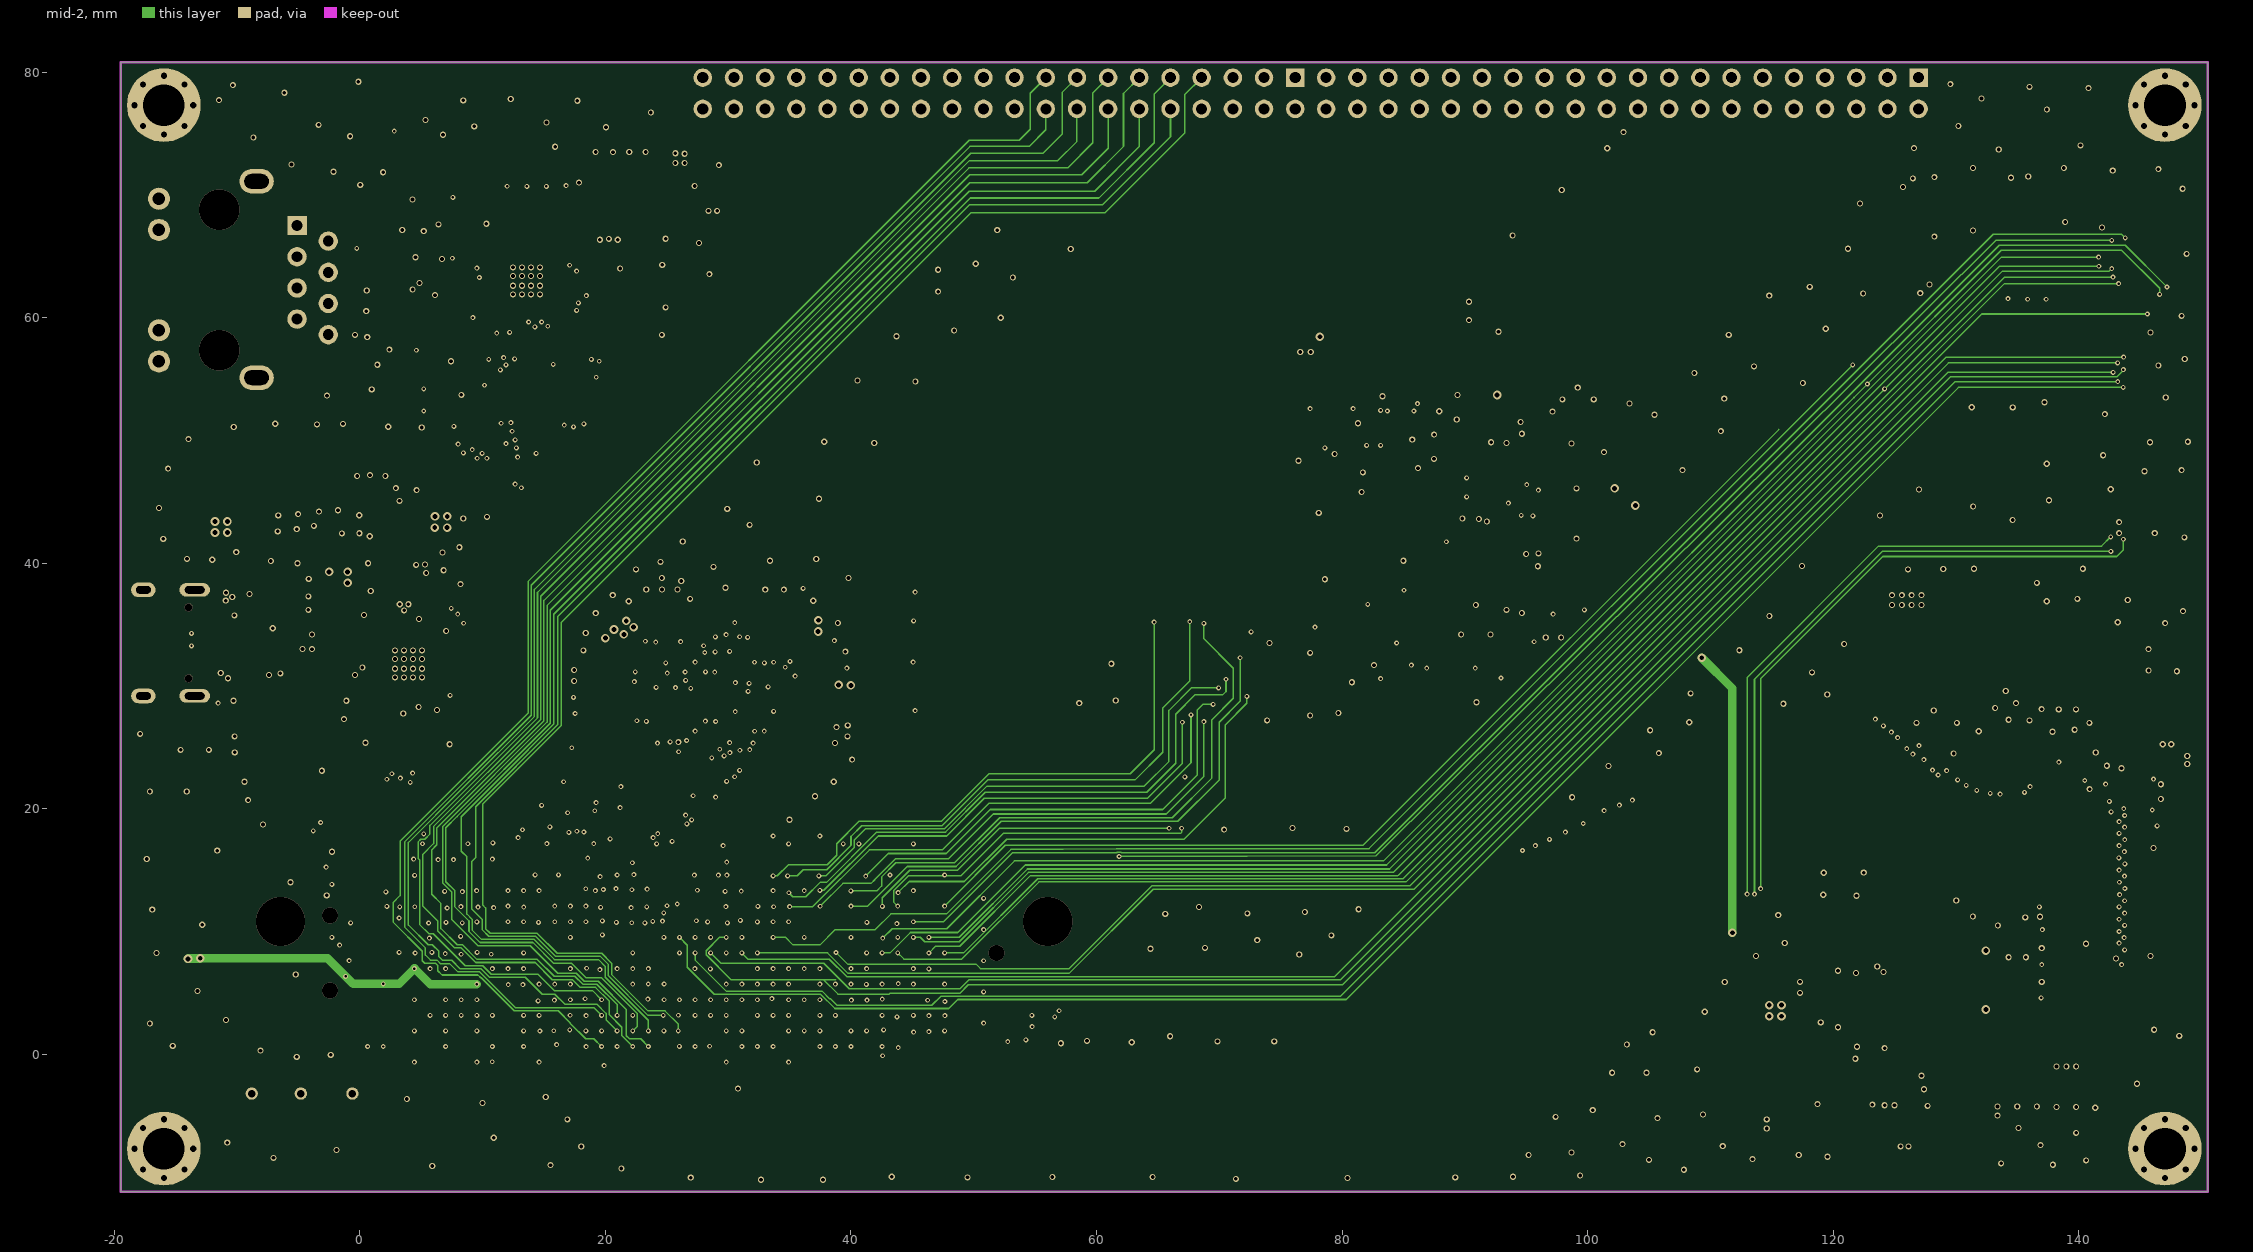
[diagram p0: mid-2]
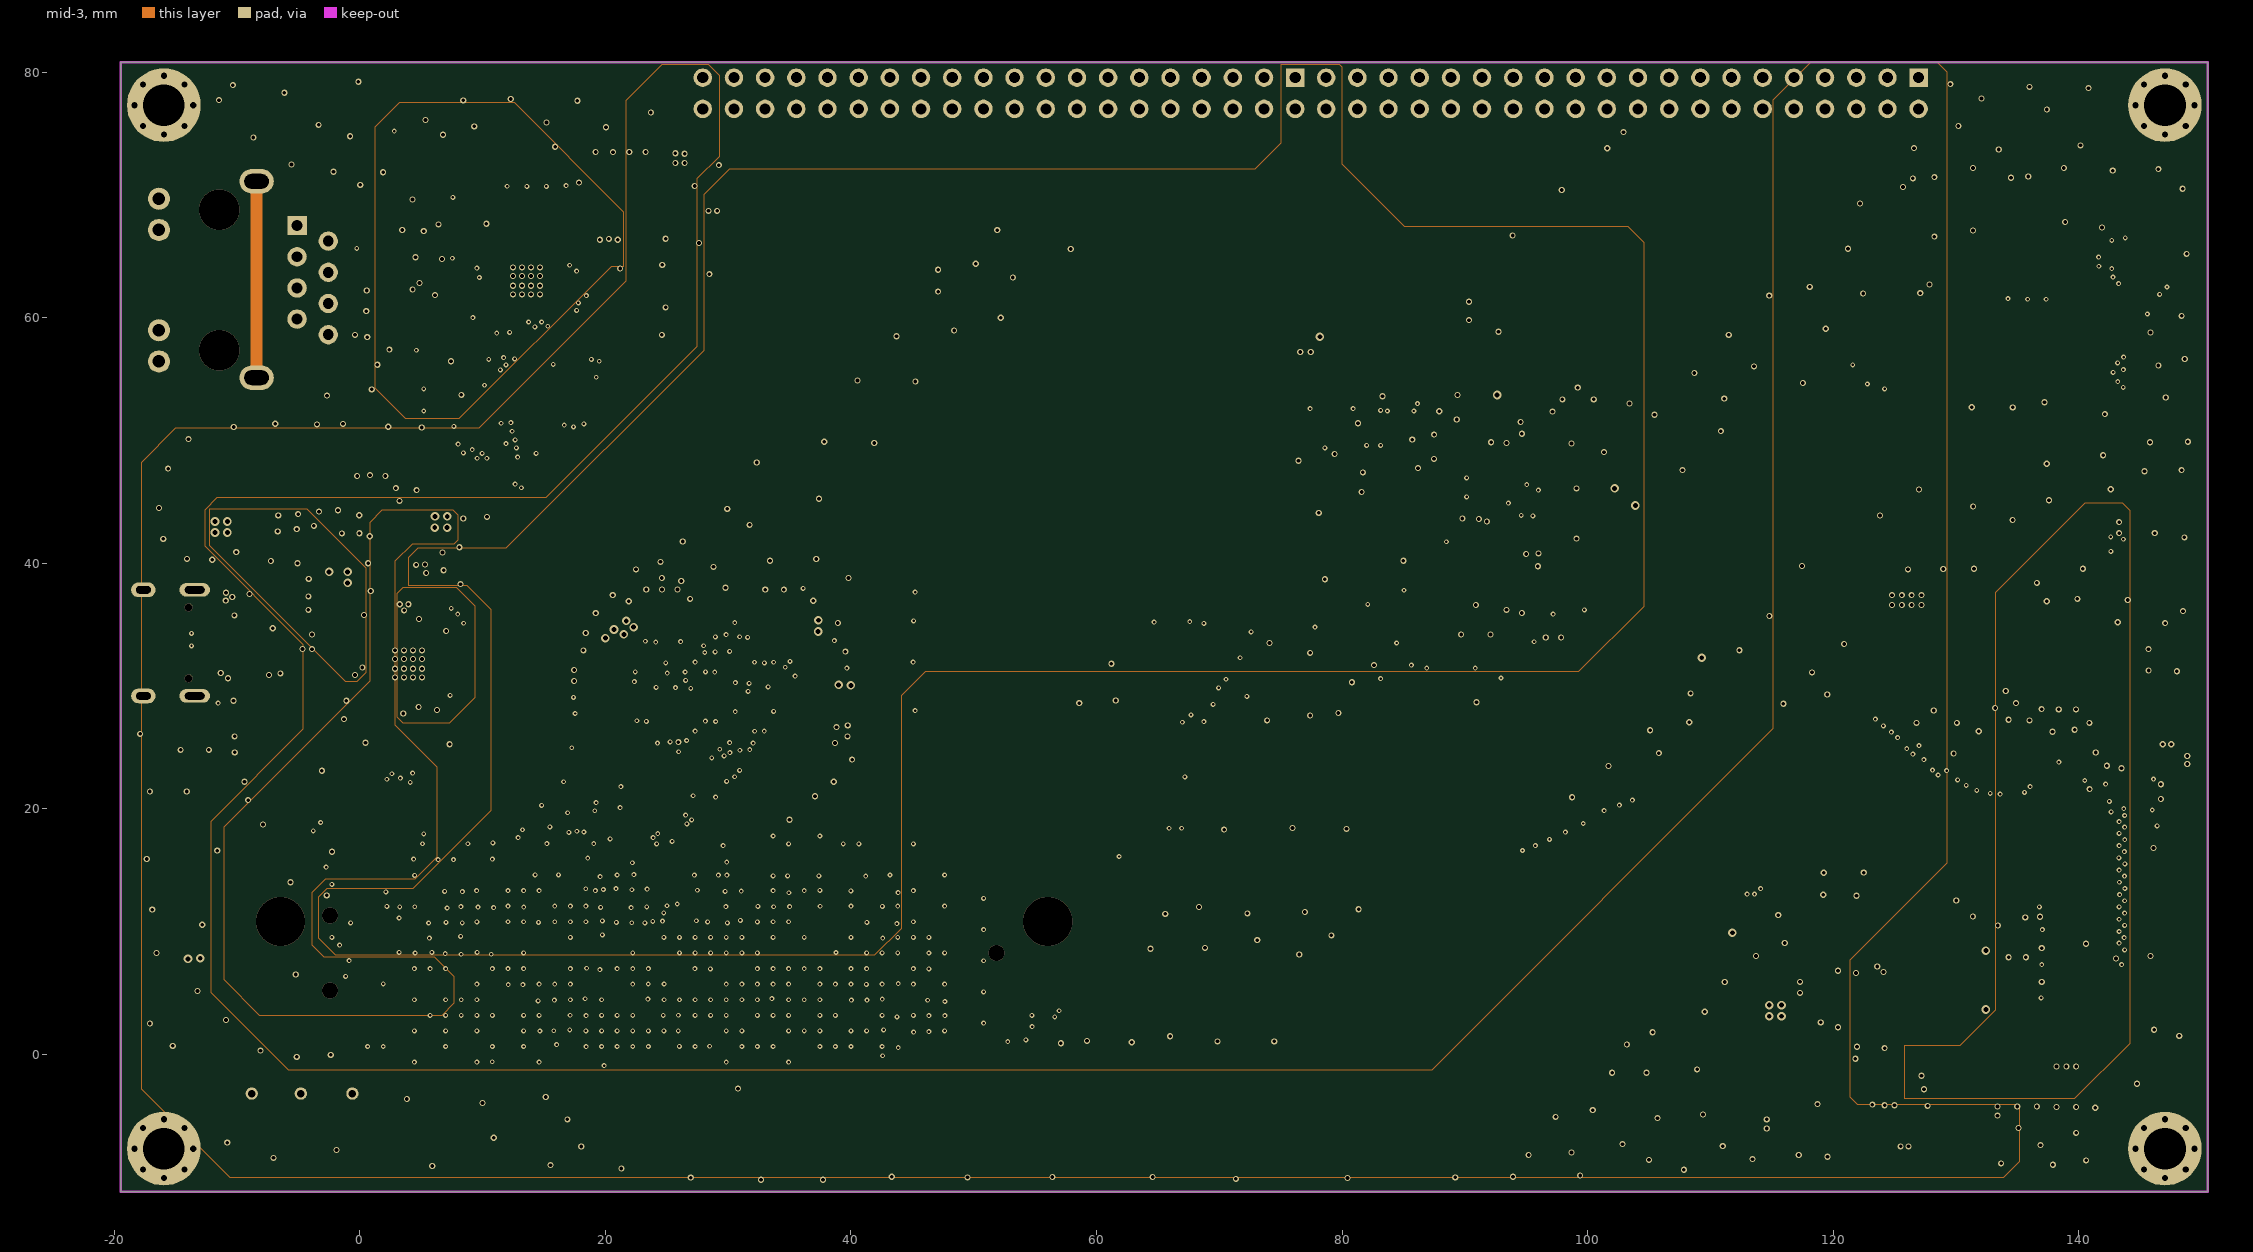
[diagram p1: mid-3]
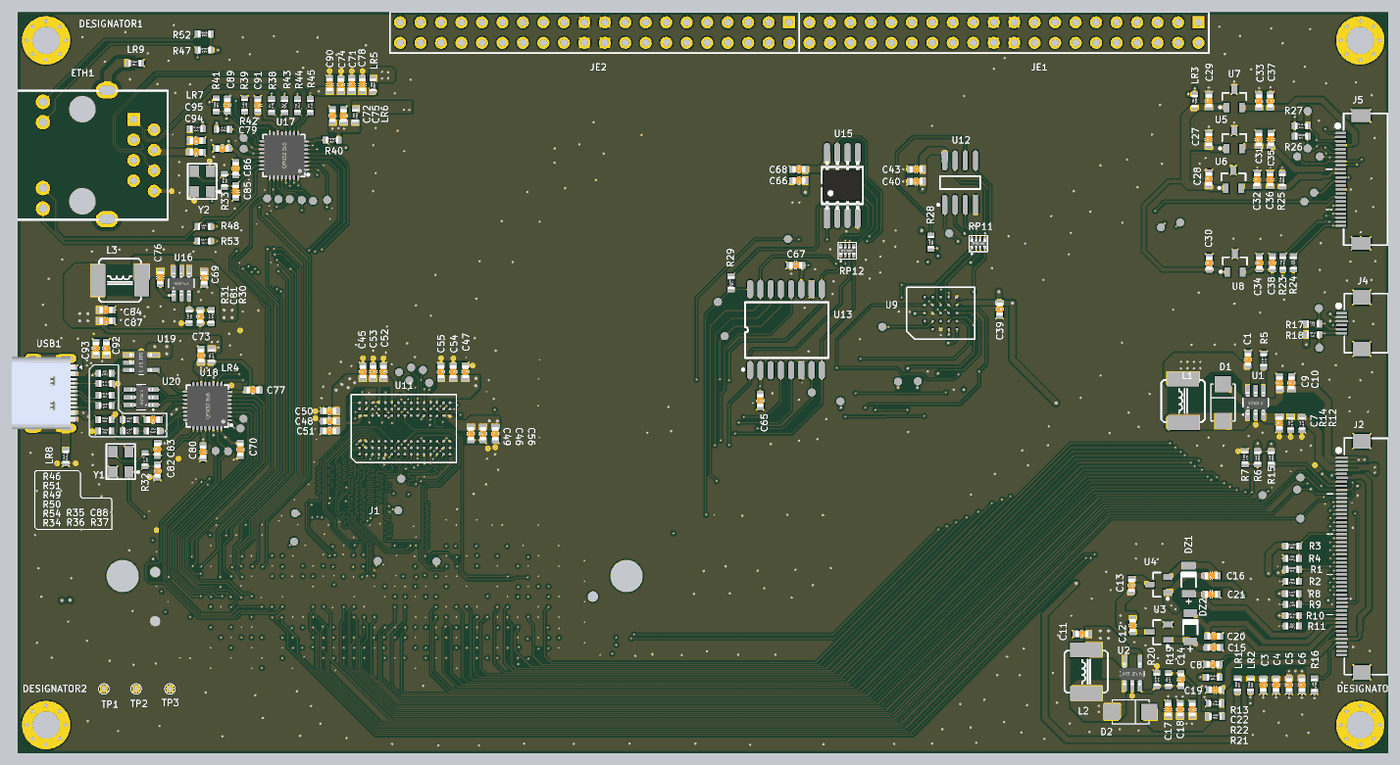
[diagram p2: 3D render of the assembled board from above, using the file's embedded part models]
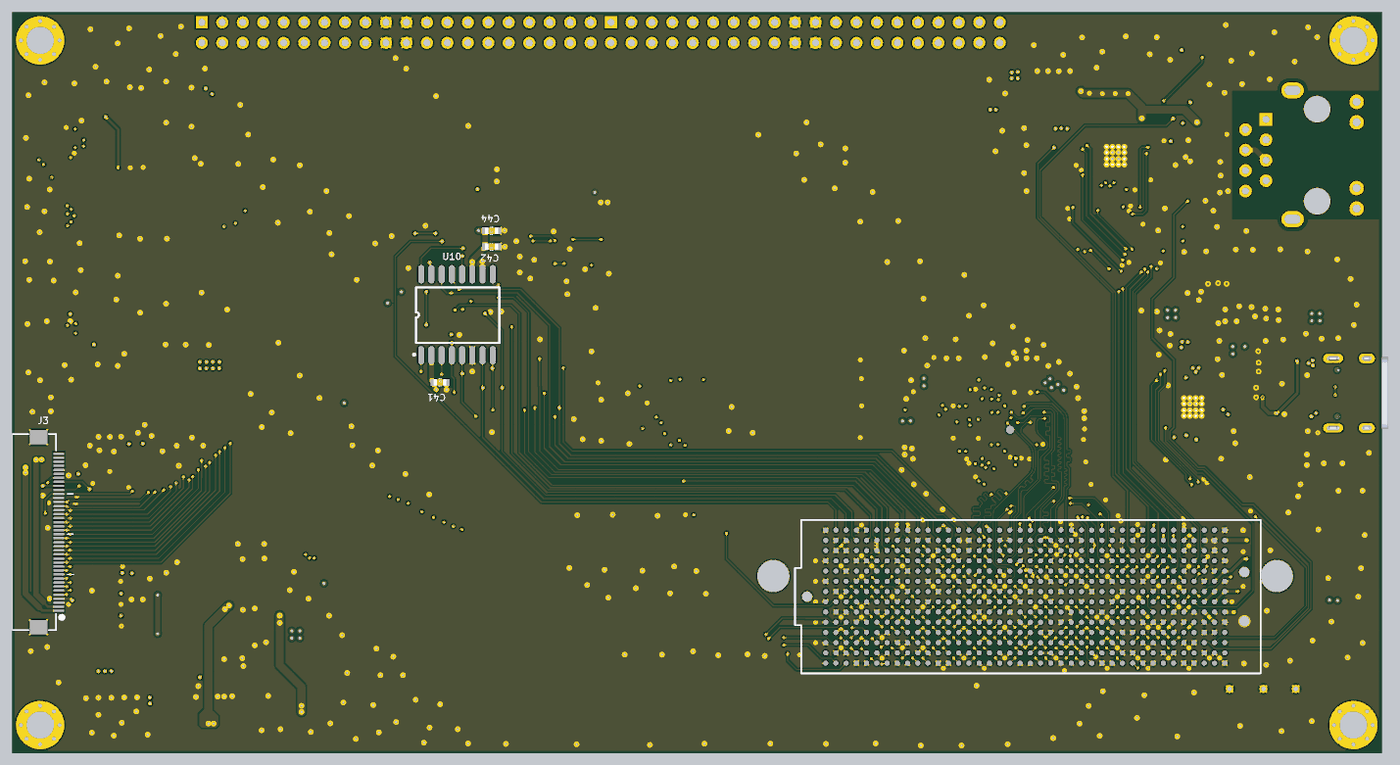
[diagram p3: 3D render of the assembled board from below, using the file's embedded part models]
# Altium PCB MISC105414.PcbDoc (part 2 of 11)
## Components (designator, comment, footprint, x,y, rotation, side; value= is the part's Value field where it differs from the comment) (continued)
C91 "0603C_N" 0603C_N 10.286,70.052 r270 top
C92 "0603C_N" 0603C_N -8.492,38.276 r90 top
C93 "0603C_N" 0603C_N -9.792,38.276 r90 top
C94 "0603C_N" 0603C_N 3.452,63.427 r180 top
C95 "0603C_N" 0603C_N 3.452,64.862 r180 top
D1 "DO-214AC" DO-214AC 130,30.05 r90 top
D2 "DO-214AC" DO-214AC 116.25,-6.05 r0 top
DESIGNATOR1 "FZ_HOLE_M3.4" FZ_HOLE_M3.4 -15.97,77.31 r0 top
DESIGNATOR2 "FZ_HOLE_M3.4" FZ_HOLE_M3.4 -15.97,-7.69 r0 top
DESIGNATOR3 "FZ_HOLE_M3.4" FZ_HOLE_M3.4 147.03,-7.69 r0 top
DESIGNATOR4 "FZ_HOLE_M3.4" FZ_HOLE_M3.4 147.03,77.31 r0 top
DZ1 "LL-34" LL-34 125.75,10.35 r90 top
DZ2 "LL-34" LL-34 125.95,4.45 r90 top
ETH1 "RJ45_HR911003A" RJ45_HR911003A -9.47,63.11 r270 top
J1 "ASP-184330-01_BOTTOM" ASP-184330-01_BOTTOM 49.53,0 r180 top
J2 "FPC0.5-50P" ?#1 144.73,1.01 r90 top
J3 "FPC0.5-40P" ?#2 144.73,26.01 r270 bottom
J4 "FPC0.5-6P" ?#3 144.733,43.46 r90 top
J5 "FPC0.5-24P" ?#4 144.63,65.81 r90 top
JE1 "HDR2X20" HDR2X20 126.97,79.55 r180 top
JE2 "HDR2X20" HDR2X20 76.19,79.55 r180 top
L1 "LD-5.5MM$2F$3" LD-5.5mm 125.05,32.55 r270 top
L2 "LD-5.5MM$2F$2" LD-5.5mm 113.029,-1.064 r270 top
L3 "LD-5.5MM" LD-5.5MM -6.814,47.528 r180 top
LR1 "0603R_N" 0603R_N 131.8,-1.9 r270 top
LR2 "0603R_N" 0603R_N 133.4,-1.9 r270 top
LR3 "0603R_N" 0603R_N 126.5,69 r90 top
LR4 "0603R_N" 0603R_N 4.566,37.397 r90 top
LR5 "0603R_N" 0603R_N 24.6,71 r90 top
LR6 "0603R_N" 0603R_N 22.4,67.2 r90 top
LR7 "0603R_N" 0603R_N 3.452,66.34 r180 top
LR8 "0603R_N" 0603R_N -13.53,24.812 r90 top
LR9 "0603R_N" 0603R_N -4.2,74.5 r180 top
R1 "0603R_N" 0603R_N 139.4,11.65 r180 top
R2 "0603R_N" 0603R_N 137.8,10.15 r0 top
R3 "0603R_N" 0603R_N 139.4,14.55 r180 top
R4 "0603R_N" 0603R_N 137.8,13 r0 top
R5 "0603R_N" 0603R_N 135.05,38.4 r270 top
R6 "0603R_N" 0603R_N 134.3,24.7 r90 top
R7 "0603R_N" 0603R_N 132.75,26.3 r270 top
R8 "0603R_N" 0603R_N 139.368,8.625 r180 top
R9 "0603R_N" 0603R_N 137.792,7.3 r0 top
R10 "0603R_N" 0603R_N 139.4,5.9 r180 top
R11 "0603R_N" 0603R_N 137.8,4.6 r0 top
R12 "0603R_N" 0603R_N 139.8,28.982 r90 top
R13 "0603R_N" 0603R_N 129.55,-1.75 r180 top
R14 "0603R_N" 0603R_N 138.4,28.982 r90 top
R15 "0603R_N" 0603R_N 136,24.7 r90 top
R16 "0603R_N" 0603R_N 141.35,-3.5 r90 top
R17 "0603R_N" 0603R_N 141.93,42.11 r180 top
R18 "0603R_N" 0603R_N 141.93,40.81 r180 top
R19 "0603R_N" 0603R_N 123.25,-2.85 r90 top
R20 "0603R_N" 0603R_N 121.8,-1.25 r270 top
R21 "0603R_N" 0603R_N 129.85,-6.6 r180 top
R22 "0603R_N" 0603R_N 128.238,-4.988 r0 top
R23 "0603R_N" 0603R_N 137.43,48.91 r90 top
R24 "0603R_N" 0603R_N 138.73,48.91 r90 top
R25 "0603R_N" 0603R_N 137.343,59.203 r90 top
R26 "0603R_N" 0603R_N 140.5,65.4 r180 top
R27 "0603R_N" 0603R_N 140.5,66.7 r180 top
R28 "0603R_N" 0603R_N 93.75,53.05 r270 top
R29 "0603R_N" 0603R_N 69,48 r270 top
R30 "0603R_N" 0603R_N 4.521,42.225 r90 top
R31 "0603R_N" 0603R_N 1.771,43.825 r270 top
R32 "0603R_N" 0603R_N -3.7,26.05 r270 top
R33 "0603R_N" 0603R_N 6.15,60.7 r270 top
R34 "0603R_N" 0603R_N -7.892,28.836 r180 top
R35 "0603R_N" 0603R_N -4.874,30.236 r180 top
R36 "0603R_N" 0603R_N -4.874,28.836 r180 top
R37 "0603R_N" 0603R_N -3.492,28.836 r0 top
R38 "0603R_N" 0603R_N 12,68.4 r90 top
R39 "0603R_N" 0603R_N 8.652,70.073 r270 top
R40 "0603R_N" 0603R_N 20.279,64.943 r180 top
R41 "0603R_N" 0603R_N 5.103,70.089 r270 top
R42 "0603R_N" 0603R_N 5.177,66.262 r0 top
R43 "0603R_N" 0603R_N 13.6,68.4 r90 top
R44 "0603R_N" 0603R_N 15.2,68.4 r90 top
R45 "0603R_N" 0603R_N 16.8,68.4 r90 top
R46 "0603R_N" 0603R_N -9.455,35.98 r0 top
R47 "0603R_N" 0603R_N 4.443,76.103 r180 top
R48 "0603R_N" 0603R_N 4.4,54.2 r180 top
R49 "0603R_N" 0603R_N -7.87,33.26 r180 top
R50 "0603R_N" 0603R_N -7.87,31.985 r180 top
R51 "0603R_N" 0603R_N -7.855,34.705 r180 top
R52 "0603R_N" 0603R_N 4.443,78.103 r180 top
R53 "0603R_N" 0603R_N 4.4,52.4 r180 top
R54 "0603R_N" 0603R_N -7.892,30.236 r180 top
RP11 "0402RP-4P" 0402RP-4P 99.65,52.1 r0 top
RP12 "0402RP-4P" 0402RP-4P 83.4,51.2 r0 top
TP1 "FZ_TP-VIA" FZ_TP-VIA -8.81,-3.2 r0 top
TP2 "FZ_TP-VIA" FZ_TP-VIA -4.81,-3.2 r0 top
TP3 "FZ_TP-VIA" FZ_TP-VIA -0.61,-3.2 r0 top
TP4 "FZ_TP-SMD-MINI" FZ_TP-SMD-MINI 139.6,23.05 r0 top
TP5 "FZ_TP-SMD-MINI" FZ_TP-SMD-MINI 139.2,21.55 r0 top
TP6 "FZ_TP-SMD-MINI" FZ_TP-SMD-MINI 139.6,17.95 r0 top
TP7 "FZ_TP-SMD-MINI" FZ_TP-SMD-MINI 134.9,20.85 r0 top
TP8 "FZ_TP-SMD-MINI" FZ_TP-SMD-MINI 141.95,39.15 r0 top
TP9 "FZ_TP-SMD-MINI" FZ_TP-SMD-MINI 141.9,44.05 r0 top
TP10 "FZ_TP-SMD-MINI" FZ_TP-SMD-MINI 142,62.9 r90 top
TP11 "FZ_TP-SMD-MINI" FZ_TP-SMD-MINI 139.2,62.9 r90 top
TP12 "FZ_TP-SMD-MINI" FZ_TP-SMD-MINI 122.3,54.1 r90 top
TP13 "FZ_TP-SMD-MINI" FZ_TP-SMD-MINI 140.5,68.55 r90 top
TP14 "FZ_TP-SMD-MINI" FZ_TP-SMD-MINI 140.5,63.9 r90 top
TP15 "FZ_TP-SMD-MINI" FZ_TP-SMD-MINI 124.7,54.7 r90 top
TP16 "FZ_TP-SMD-MINI" FZ_TP-SMD-MINI 141.3,58.4 r90 top
TP17 "FZ_TP-SMD-MINI" FZ_TP-SMD-MINI 140.1,57.3 r90 top
TP18 "FZ_TP-SMD-MINI" FZ_TP-SMD-MINI 89.7,34.95 r90 top
TP19 "FZ_TP-SMD-MINI" FZ_TP-SMD-MINI 87.75,41.75 r90 top
TP20 "FZ_TP-SMD-MINI" FZ_TP-SMD-MINI 82.55,32.5 r90 top
TP21 "FZ_TP-SMD-MINI" FZ_TP-SMD-MINI 92.15,35 r270 top
TP22 "FZ_TP-SMD-MINI" FZ_TP-SMD-MINI 14.902,18.61 r90 top
TP23 "FZ_TP-SMD-MINI" FZ_TP-SMD-MINI 14.783,15.095 r90 top
TP24 "FZ_TP-SMD-MINI" FZ_TP-SMD-MINI 27.81,36.126 r90 top
TP25 "FZ_TP-SMD-MINI" FZ_TP-SMD-MINI 31.545,34.807 r90 top
TP26 "FZ_TP-SMD-MINI" FZ_TP-SMD-MINI 30.77,36.392 r90 top
TP27 "FZ_TP-SMD-MINI" FZ_TP-SMD-MINI 29.077,35.099 r90 top
TP28 "FZ_TP-SMD-MINI" FZ_TP-SMD-MINI 29.312,36.708 r90 top
TP29 "FZ_TP-SMD-MINI" FZ_TP-SMD-MINI 27.704,18.966 r90 top
TP30 "FZ_TP-SMD-MINI" FZ_TP-SMD-MINI 26.646,28.973 r90 bottom
TP31 "FZ_TP-SMD-MINI" FZ_TP-SMD-MINI 25.166,12.691 r90 top
TP32 "FZ_TP-SMD-MINI" FZ_TP-SMD-MINI 28.084,22.885 r90 top
TP33 "FZ_TP-SMD-MINI" FZ_TP-SMD-MINI 32.453,12.631 r90 top
TP34 "FZ_TP-SMD-MINI" FZ_TP-SMD-MINI 96.05,53.35 r90 top
TP35 "FZ_TP-SMD-MINI" FZ_TP-SMD-MINI 79,33.6 r90 top
TP36 "FZ_TP-SMD-MINI" FZ_TP-SMD-MINI 67.35,44.85 r90 top
TP37 "FZ_TP-SMD-MINI" FZ_TP-SMD-MINI 68.2,40.6 r90 top
TP39 "FZ_TP-SMD-MINI" FZ_TP-SMD-MINI 76.05,52.65 r90 top
TP40 "FZ_TP-SMD-MINI" FZ_TP-SMD-MINI 18.9,57.5 r90 top
TP41 "FZ_TP-SMD-MINI" FZ_TP-SMD-MINI 12.845,57.586 r90 top
TP42 "FZ_TP-SMD-MINI" FZ_TP-SMD-MINI 15.745,57.486 r90 top
TP43 "FZ_TP-SMD-MINI" FZ_TP-SMD-MINI 11.445,57.686 r90 top
TP44 "FZ_TP-SMD-MINI" FZ_TP-SMD-MINI 17.145,57.386 r90 top
TP45 "FZ_TP-SMD-MINI" FZ_TP-SMD-MINI 14.245,57.586 r90 top
TP46 "FZ_TP-SMD-MINI" FZ_TP-SMD-MINI 5.05,26.35 r270 top
TP47 "FZ_TP-SMD-MINI" FZ_TP-SMD-MINI 8.5,30.35 r270 top
TP48 "FZ_TP-SMD-MINI" FZ_TP-SMD-MINI 6.6,26.3 r270 top
TP49 "FZ_TP-SMD-MINI" FZ_TP-SMD-MINI 8.14,29.149 r270 top
TP50 "FZ_TP-SMD-MINI" FZ_TP-SMD-MINI 8.521,65.198 r90 top
TP51 "FZ_TP-SMD-MINI" FZ_TP-SMD-MINI 8.533,63.866 r90 top
U1 "SOT-23-6" SOT-23-6 133.1,30.85 r90 top
U2 "SOT-23-5" SOT-23-5 118.75,-1.3 r90 top
U3 "SOT-23" SOT-23 122.05,3.85 r90 top
U4 "SOT-23" SOT-23 122.05,9.75 r90 top
U5 "SOT-23" SOT-23 131.4,65 r0 top
U6 "SOT-23" SOT-23 131.3,60.1 r0 top
U7 "SOT-23" SOT-23 131.4,70.1 r0 top
U8 "SOT-23" SOT-23 131.484,49.686 r0 top
U9 "PBGA24_6X8" PBGA24_6X8 94.297,41.232 r90 top
U10 "SOIC16" SOIC16 95.3,43.25 r90 bottom
U11 "VFBGA90_8X13" VFBGA90_8X13 28.52,29.133 r90 top
U12 "SOP8" SOP8 97.4,59.65 r90 top
U13 "SOIC16" SOIC16 75.8,41.4 r90 top
U15 "SOIC8" SOIC8 82.8,59.3 r90 top
U16 "SOT-23-6" SOT-23-6 -0.138,45.661 r90 top
U17 "QFN32_5X5$2F$2" "QFN32 5X5" 13.53,63.01 r90 top
U18 "QFN32_5X5" "QFN32 5X5" 4.03,31.91 r90 top
U19 "SOT-23-5" SOT-23-5 -4.161,37.317 r0 top
U20 "SOT-23-6" SOT-23-6 -2.67,32.06 r180 top
USB1 "USB_TYPE-C_16PIN" USB_TYPE-C_16PIN -15.17,33.51 r180 top
Y1 "XTAL_SMD3225$2F$2" XTAL_SMD3225$2F$2 -6.7,25 r90 top
Y2 "XTAL_SMD3225" XTAL_SMD3225 3.4,59.8 r90 top

## Footprints (in the part's own frame and the unit in brackets; to place one, negate y for a bottom-side part, rotate by r counter-clockwise, add the part's x,y. Pads: shape width x height; smd on the part's side, far side on the other; paste and mask are expansions set on the pad)
0402RP-4P [mm] "2mm*1mm*0.45mm(长*宽*厚)"
  rect 0.4x0.6 smd: 1(-0.8,-0.5) 4(0.8,-0.5) 5(0.8,0.5) 8(-0.8,0.5)
  rect 0.3x0.6 smd: 2(-0.25,-0.5) 3(0.25,-0.5) 6(0.25,0.5) 7(-0.25,0.5)
  silkscreen extent -1.14,-1.38 1.15,1.01, body extent -1,-0.5 1,0.5, height 0.45
0603C_N [mil]
  rect 30x34 smd: 1(0,-0.01) 2(62.99,-0.01)
  Top pour cut-out: 15.74,25 47.24,25 47.24,-25 15.74,-25
  silkscreen extent 22,-17 40,18, body extent 0,-16 63,16, height 12
0603R_N [mil]
  rect 30x34 smd: 1(0,0) 2(62.99,0)
  Top pour cut-out: 19,-25 19,25 44,25 44,-25
  body extent 0,-17 61,17, height 18